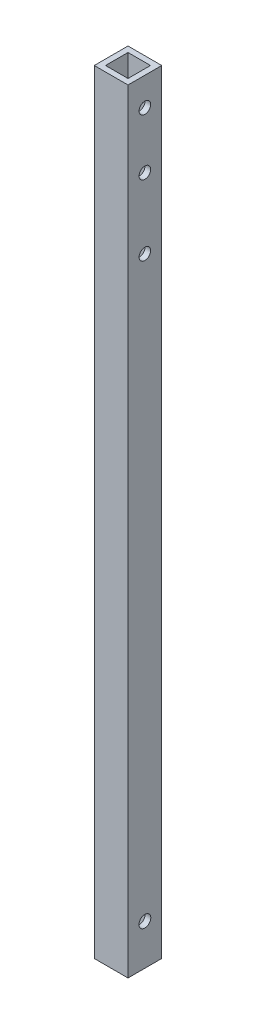
SolidWorks part; units mm, degrees
material "Thornel Mat VMA"
ref_plane "前视基准面" through (0, 0, 0) normal (0, 0, 1) x (1, 0, 0)
ref_plane "上视基准面" through (0, 0, 0) normal (0, 1, 0) x (1, 0, 0)
ref_plane "右视基准面" through (0, 0, 0) normal (1, 0, 0) x (0, 0, -1)
sketch "草图1" plane through (0, 0, 0) normal (0, 1, 0) x (1, 0, 0)
  line L1 (-4, 4) -> (4, 4)
  line L2 (-4, 4) -> (-4, -4)
  line L3 (-4, -4) -> (4, -4)
  line L4 (4, 4) -> (4, -4)
  line L5 (-4, 4) -> (4, -4) construction
  line L6 (-4, -4) -> (4, 4) construction
  line L7 (-6, 6) -> (6, 6)
  line L8 (-6, 6) -> (-6, -6)
  line L9 (-6, -6) -> (6, -6)
  line L10 (6, 6) -> (6, -6)
  line L11 (-6, 6) -> (6, -6) construction
  line L12 (-6, -6) -> (6, 6) construction
  point P0 (0, 0)
  point P5 (0, 0)
  dimension "D1" = 2
  dimension "D2" = 12
extrude "凸台-拉伸1" add sketch "草图1" along normal blind 275
sketch "草图2" plane through (0, 0, 6) normal (0, 0, 1) x (1, 0, 0)
  line L0 (0, 26.5) -> (0, 6.5) construction
  line L1 (-6, 0) -> (6, 0) construction
  circle A0 centre (0, 6.5) radius 2.1
  circle A1 centre (0, 26.5) radius 2.1
  dimension "D1" = 4.2
  dimension "D2" = 6.5
  dimension "D3" = 20
extrude "切除-拉伸1" [suppressed] cut sketch "草图2" against normal through all
sketch "草图3" plane through (-6, 0, 0) normal (-1, 0, 0) x (0, 0, 1)
  line L1 (0, 265) -> (0, 220) construction
  line L2 (6, 275) -> (6, 0) construction
  line L3 (-6, 275) -> (-6, 0) construction
  line L4 (-6, 275) -> (6, 275) construction
  line L6 (-6, 0) -> (6, 0) construction
  circle A2 centre (0, 265) radius 2.05
  circle A3 centre (0, 245) radius 2.05
  circle A4 centre (0, 220) radius 2.05
  circle A5 centre (0, 14.5) radius 2.1
  point P20 (-52.3802, 30.5979)
  dimension "D1" = 4.1
  dimension "D2" = 10
  dimension "D3" = 45
  dimension "D4" = 20
  dimension "D5" = 4.2
  dimension "D6" = 14.5
extrude "切除-拉伸2" cut sketch "草图3" against normal through all
sketch "草图4" [suppressed] plane through (-6, 0, 0) normal (-1, 0, 0) x (0, 0, 1)
  line L0 (0, 275) -> (0, 0) construction
  line L1 (-6, 275) -> (6, 275) construction
  line L2 (-0.4696, 207.7652) -> (-2.4196, 206.7902)
  line L3 (-3, 205.8511) -> (-3, 201.1989)
  line L4 (-1.4804, 200.2598) -> (-0.4696, 200.7652)
  line L5 (0.4696, 200.7652) -> (1.4804, 200.2598)
  line L6 (3, 201.1989) -> (3, 205.8511)
  line L7 (2.4196, 206.7902) -> (0.4696, 207.7652)
  line L8 (2.4196, 186.7902) -> (0.4696, 187.7652)
  line L9 (-0.4696, 187.7652) -> (-2.4196, 186.7902)
  line L10 (-3, 185.8511) -> (-3, 181.1989)
  line L11 (-1.4804, 180.2598) -> (-0.4696, 180.7652)
  line L12 (0.4696, 180.7652) -> (1.4804, 180.2598)
  line L13 (3, 181.1989) -> (3, 185.8511)
  line L14 (2.4196, 166.7902) -> (0.4696, 167.7652)
  line L15 (-0.4696, 167.7652) -> (-2.4196, 166.7902)
  line L16 (-3, 165.8511) -> (-3, 161.1989)
  line L17 (-1.4804, 160.2598) -> (-0.4696, 160.7652)
  line L18 (0.4696, 160.7652) -> (1.4804, 160.2598)
  line L19 (3, 161.1989) -> (3, 165.8511)
  line L20 (2.4196, 146.7902) -> (0.4696, 147.7652)
  line L21 (-0.4696, 147.7652) -> (-2.4196, 146.7902)
  line L22 (-3, 145.8511) -> (-3, 141.1989)
  line L23 (-1.4804, 140.2598) -> (-0.4696, 140.7652)
  line L24 (0.4696, 140.7652) -> (1.4804, 140.2598)
  line L25 (3, 141.1989) -> (3, 145.8511)
  line L26 (2.4196, 126.7902) -> (0.4696, 127.7652)
  line L27 (-0.4696, 127.7652) -> (-2.4196, 126.7902)
  line L28 (-3, 125.8511) -> (-3, 121.1989)
  line L29 (-1.4804, 120.2598) -> (-0.4696, 120.7652)
  line L30 (0.4696, 120.7652) -> (1.4804, 120.2598)
  line L31 (3, 121.1989) -> (3, 125.8511)
  line L32 (2.4196, 106.7902) -> (0.4696, 107.7652)
  line L33 (-0.4696, 107.7652) -> (-2.4196, 106.7902)
  line L34 (-3, 105.8511) -> (-3, 101.1989)
  line L35 (-1.4804, 100.2598) -> (-0.4696, 100.7652)
  line L36 (0.4696, 100.7652) -> (1.4804, 100.2598)
  line L37 (3, 101.1989) -> (3, 105.8511)
  line L38 (2.4196, 86.7902) -> (0.4696, 87.7652)
  line L39 (-0.4696, 87.7652) -> (-2.4196, 86.7902)
  line L40 (-3, 85.8511) -> (-3, 81.1989)
  line L41 (-1.4804, 80.2598) -> (-0.4696, 80.7652)
  line L42 (0.4696, 80.7652) -> (1.4804, 80.2598)
  line L43 (3, 81.1989) -> (3, 85.8511)
  line L44 (2.4196, 66.7902) -> (0.4696, 67.7652)
  line L45 (-0.4696, 67.7652) -> (-2.4196, 66.7902)
  line L46 (-3, 65.8511) -> (-3, 61.1989)
  line L47 (-1.4804, 60.2598) -> (-0.4696, 60.7652)
  line L48 (0.4696, 60.7652) -> (1.4804, 60.2598)
  line L49 (3, 61.1989) -> (3, 65.8511)
  line L50 (2.4196, 46.7902) -> (0.4696, 47.7652)
  line L51 (-0.4696, 47.7652) -> (-2.4196, 46.7902)
  line L52 (-3, 45.8511) -> (-3, 41.1989)
  line L53 (-1.4804, 40.2598) -> (-0.4696, 40.7652)
  line L54 (0.4696, 40.7652) -> (1.4804, 40.2598)
  line L55 (3, 41.1989) -> (3, 45.8511)
  circle A0 centre (0, 220) radius 2.05 construction
  arc A1 (-0.4696, 200.7652) -> (0.4696, 200.7652) centre (0, 199.8261) cw
  arc A2 (1.4804, 200.2598) -> (3, 201.1989) centre (1.95, 201.1989) ccw
  arc A3 (3, 205.8511) -> (2.4196, 206.7902) centre (1.95, 205.8511) ccw
  arc A4 (-0.4696, 207.7652) -> (0.4696, 207.7652) centre (0, 206.8261) cw
  arc A5 (-3, 201.1989) -> (-1.4804, 200.2598) centre (-1.95, 201.1989) ccw
  arc A6 (-2.4196, 206.7902) -> (-3, 205.8511) centre (-1.95, 205.8511) ccw
  arc A7 (-0.4696, 187.7652) -> (0.4696, 187.7652) centre (0, 186.8261) cw
  arc A8 (3, 185.8511) -> (2.4196, 186.7902) centre (1.95, 185.8511) ccw
  arc A9 (-2.4196, 186.7902) -> (-3, 185.8511) centre (-1.95, 185.8511) ccw
  arc A10 (-3, 181.1989) -> (-1.4804, 180.2598) centre (-1.95, 181.1989) ccw
  arc A11 (-0.4696, 180.7652) -> (0.4696, 180.7652) centre (0, 179.8261) cw
  arc A12 (1.4804, 180.2598) -> (3, 181.1989) centre (1.95, 181.1989) ccw
  arc A13 (-0.4696, 167.7652) -> (0.4696, 167.7652) centre (0, 166.8261) cw
  arc A14 (3, 165.8511) -> (2.4196, 166.7902) centre (1.95, 165.8511) ccw
  arc A15 (-2.4196, 166.7902) -> (-3, 165.8511) centre (-1.95, 165.8511) ccw
  arc A16 (-3, 161.1989) -> (-1.4804, 160.2598) centre (-1.95, 161.1989) ccw
  arc A17 (-0.4696, 160.7652) -> (0.4696, 160.7652) centre (0, 159.8261) cw
  arc A18 (1.4804, 160.2598) -> (3, 161.1989) centre (1.95, 161.1989) ccw
  arc A19 (-0.4696, 147.7652) -> (0.4696, 147.7652) centre (0, 146.8261) cw
  arc A20 (3, 145.8511) -> (2.4196, 146.7902) centre (1.95, 145.8511) ccw
  arc A21 (-2.4196, 146.7902) -> (-3, 145.8511) centre (-1.95, 145.8511) ccw
  arc A22 (-3, 141.1989) -> (-1.4804, 140.2598) centre (-1.95, 141.1989) ccw
  arc A23 (-0.4696, 140.7652) -> (0.4696, 140.7652) centre (0, 139.8261) cw
  arc A24 (1.4804, 140.2598) -> (3, 141.1989) centre (1.95, 141.1989) ccw
  arc A25 (-0.4696, 127.7652) -> (0.4696, 127.7652) centre (0, 126.8261) cw
  arc A26 (3, 125.8511) -> (2.4196, 126.7902) centre (1.95, 125.8511) ccw
  arc A27 (-2.4196, 126.7902) -> (-3, 125.8511) centre (-1.95, 125.8511) ccw
  arc A28 (-3, 121.1989) -> (-1.4804, 120.2598) centre (-1.95, 121.1989) ccw
  arc A29 (-0.4696, 120.7652) -> (0.4696, 120.7652) centre (0, 119.8261) cw
  arc A30 (1.4804, 120.2598) -> (3, 121.1989) centre (1.95, 121.1989) ccw
  arc A31 (-0.4696, 107.7652) -> (0.4696, 107.7652) centre (0, 106.8261) cw
  arc A32 (3, 105.8511) -> (2.4196, 106.7902) centre (1.95, 105.8511) ccw
  arc A33 (-2.4196, 106.7902) -> (-3, 105.8511) centre (-1.95, 105.8511) ccw
  arc A34 (-3, 101.1989) -> (-1.4804, 100.2598) centre (-1.95, 101.1989) ccw
  arc A35 (-0.4696, 100.7652) -> (0.4696, 100.7652) centre (0, 99.8261) cw
  arc A36 (1.4804, 100.2598) -> (3, 101.1989) centre (1.95, 101.1989) ccw
  arc A37 (-0.4696, 87.7652) -> (0.4696, 87.7652) centre (0, 86.8261) cw
  arc A38 (3, 85.8511) -> (2.4196, 86.7902) centre (1.95, 85.8511) ccw
  arc A39 (-2.4196, 86.7902) -> (-3, 85.8511) centre (-1.95, 85.8511) ccw
  arc A40 (-3, 81.1989) -> (-1.4804, 80.2598) centre (-1.95, 81.1989) ccw
  arc A41 (-0.4696, 80.7652) -> (0.4696, 80.7652) centre (0, 79.8261) cw
  arc A42 (1.4804, 80.2598) -> (3, 81.1989) centre (1.95, 81.1989) ccw
  arc A43 (-0.4696, 67.7652) -> (0.4696, 67.7652) centre (0, 66.8261) cw
  arc A44 (3, 65.8511) -> (2.4196, 66.7902) centre (1.95, 65.8511) ccw
  arc A45 (-2.4196, 66.7902) -> (-3, 65.8511) centre (-1.95, 65.8511) ccw
  arc A46 (-3, 61.1989) -> (-1.4804, 60.2598) centre (-1.95, 61.1989) ccw
  arc A47 (-0.4696, 60.7652) -> (0.4696, 60.7652) centre (0, 59.8261) cw
  arc A48 (1.4804, 60.2598) -> (3, 61.1989) centre (1.95, 61.1989) ccw
  arc A49 (-0.4696, 47.7652) -> (0.4696, 47.7652) centre (0, 46.8261) cw
  arc A50 (3, 45.8511) -> (2.4196, 46.7902) centre (1.95, 45.8511) ccw
  arc A51 (-2.4196, 46.7902) -> (-3, 45.8511) centre (-1.95, 45.8511) ccw
  arc A52 (-3, 41.1989) -> (-1.4804, 40.2598) centre (-1.95, 41.1989) ccw
  arc A53 (-0.4696, 40.7652) -> (0.4696, 40.7652) centre (0, 39.8261) cw
  arc A54 (1.4804, 40.2598) -> (3, 41.1989) centre (1.95, 41.1989) ccw
  point P16 (0, 201)
  point P19 (3, 199.5)
  point P22 (3, 206.5)
  point P25 (0, 208)
  dimension "D4" = 12
  dimension "D5" = 1.05
  dimension "D1" = 6
  dimension "D2" = 7
  dimension "D3" = 1.5
  dimension "D7" = 20
  dimension "D6" = 9
extrude "切除-拉伸3" [suppressed] cut sketch "草图4" against normal through all
